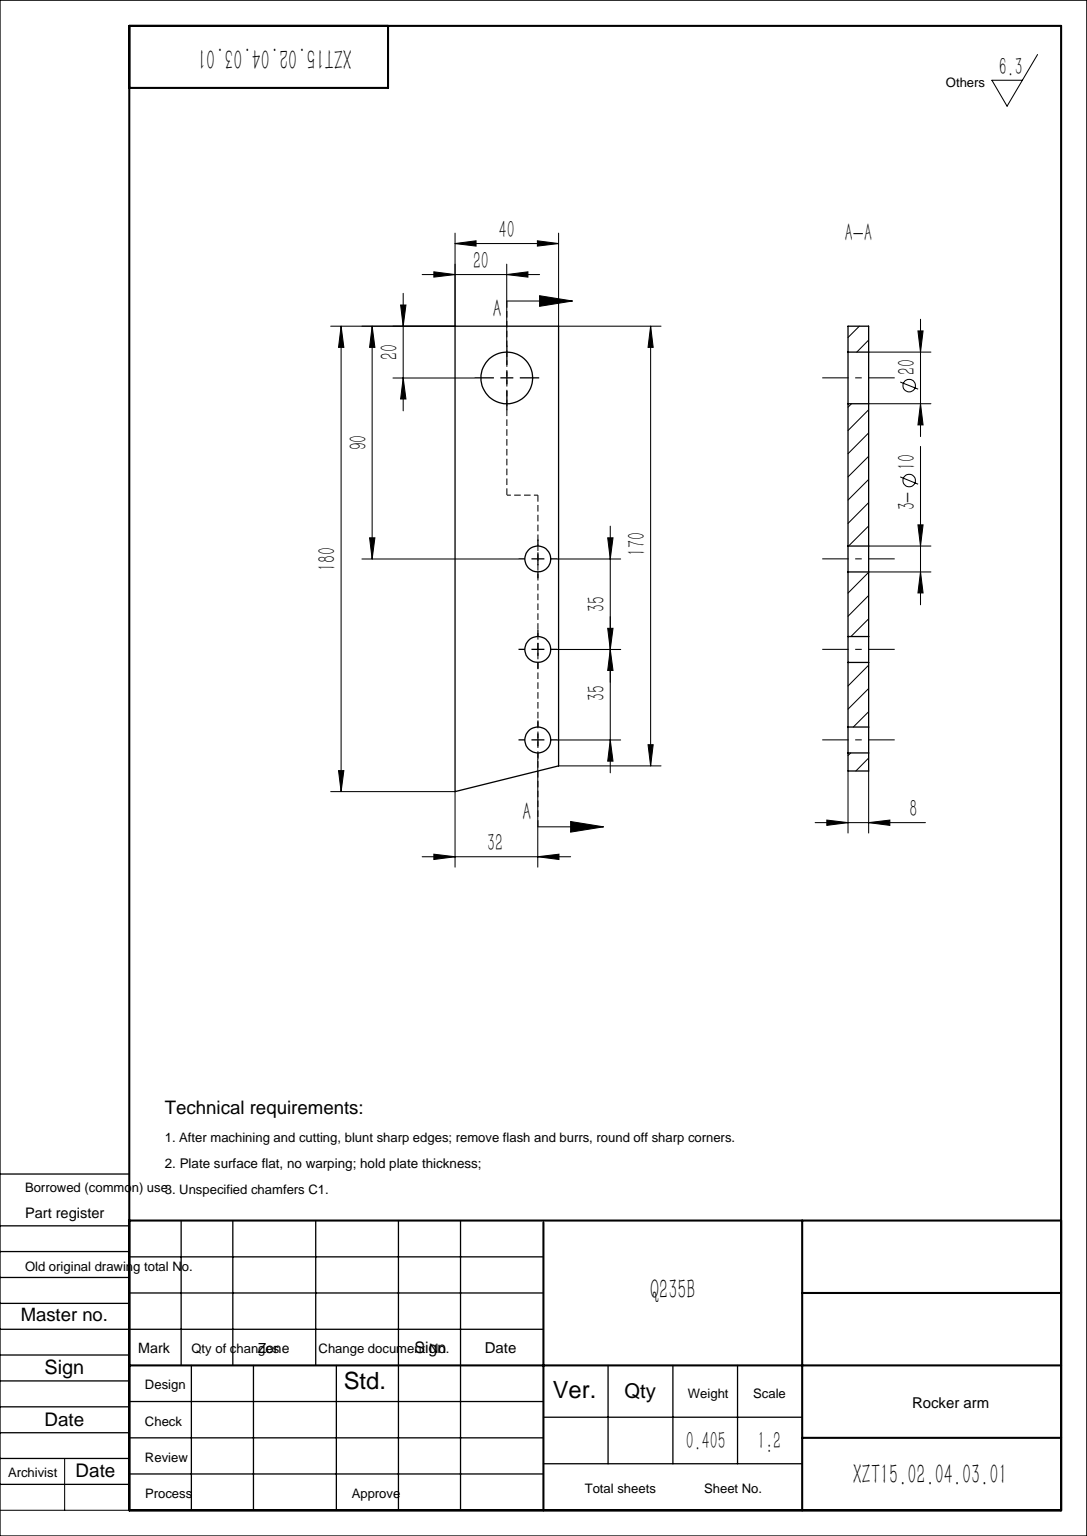
from build123d import *

# Parameters (mm, degrees)
SKETCH1_R           = 10
SKETCH1_R_2         = 5
BOSS_EXTRUDE1_DEPTH = 4


with BuildPart() as part:
    # Sketch1 → Boss-Extrude1 (new, symmetric)
    with BuildSketch(Plane.XY):
        Polygon((0, 0), (0, 180), (40, 180), (40, 10), align=None)
        with Locations((20, 160)):
            Circle(SKETCH1_R, mode=Mode.SUBTRACT)
        with Locations((32, 90)):
            Circle(SKETCH1_R_2, mode=Mode.SUBTRACT)
        with Locations((32, 55)):
            Circle(SKETCH1_R_2, mode=Mode.SUBTRACT)
        with Locations((32, 20)):
            Circle(SKETCH1_R_2, mode=Mode.SUBTRACT)
    extrude(amount=BOSS_EXTRUDE1_DEPTH, both=True)


solid = part.part
